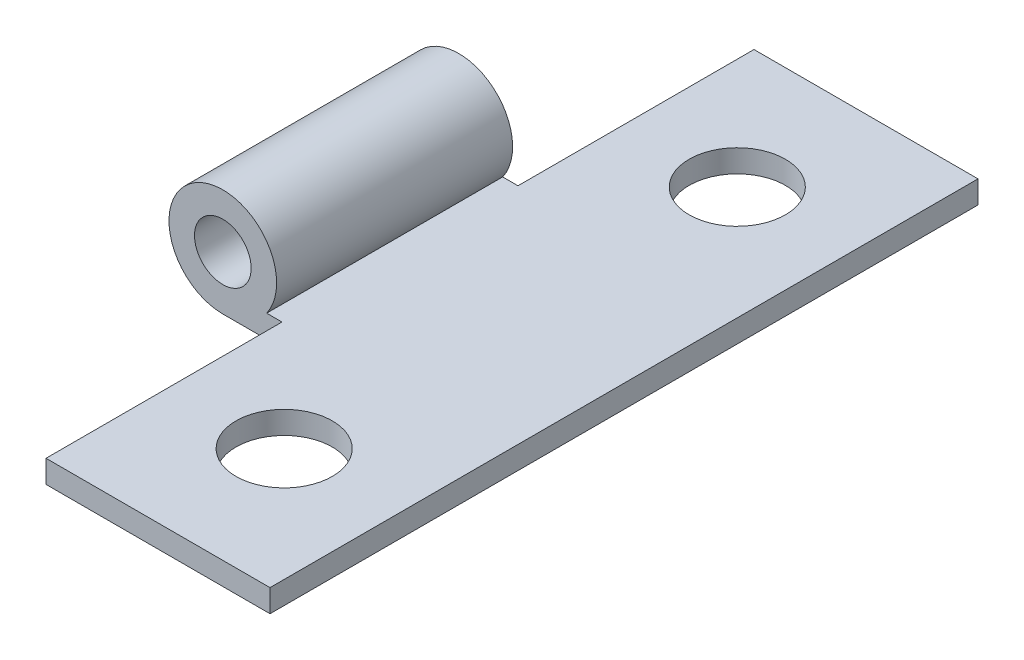
from build123d import *

# Parameters (mm, degrees)
SKETCH_1_R          = 1
EXTRUDE_1_DEPTH     = 25
CUT_EXTRUDE_1_DEPTH = 3.8
SKETCH_3_R          = 1.7
CUT_EXTRUDE_2_DEPTH = 0.8
SKETCH_4_R          = 1.7
CUT_EXTRUDE_3_DEPTH = 0.8


with BuildPart() as part:
    # 草图1 → 凸台-拉伸1 (new body)
    with BuildSketch(Plane.XY):
        with BuildLine():
            Line((0, 0), (10, 0))
            Line((10, 0), (10, 0.8))
            Line((10, 0.8), (1.549193338, 0.8))
            ThreePointArc((1.549193338, 0.8), (-0.871779789, 3.588194302), (0, 0))
        make_face()
        with Locations((0, 1.9)):
            Circle(SKETCH_1_R, mode=Mode.SUBTRACT)
    extrude(amount=-EXTRUDE_1_DEPTH)

    # 草图2 → 切除-拉伸1 (cut)
    with BuildSketch(Plane(origin=(0, 0, 0), x_dir=(1, 0, 0), z_dir=(0, 1, 0))):
        Polygon((-6, 0), (2.09, 0), (2.09, 8.333333333), (-2.09, 8.333333333), (-2.09, 16.666666667), (2.09, 16.666666667), (2.09, 25), (-6, 25), align=None)
    extrude(amount=CUT_EXTRUDE_1_DEPTH, mode=Mode.SUBTRACT)

    # 草图3 → 切除-拉伸2 (cut)
    with BuildSketch(Plane(origin=(0, 0, 0), x_dir=(1, 0, 0), z_dir=(0, 1, 0))):
        with Locations(Location((6, 20.5, 0), (0, 0, 270))):
            Circle(SKETCH_3_R)
    extrude(amount=CUT_EXTRUDE_2_DEPTH, mode=Mode.SUBTRACT)

    # 草图4 → 切除-拉伸3 (cut)
    with BuildSketch(Plane(origin=(0, 0, 0), x_dir=(1, 0, 0), z_dir=(0, 1, 0))):
        with Locations(Location((6, 4.5, 0), (0, 0, 270))):
            Circle(SKETCH_4_R)
    extrude(amount=CUT_EXTRUDE_3_DEPTH, mode=Mode.SUBTRACT)


solid = part.part
